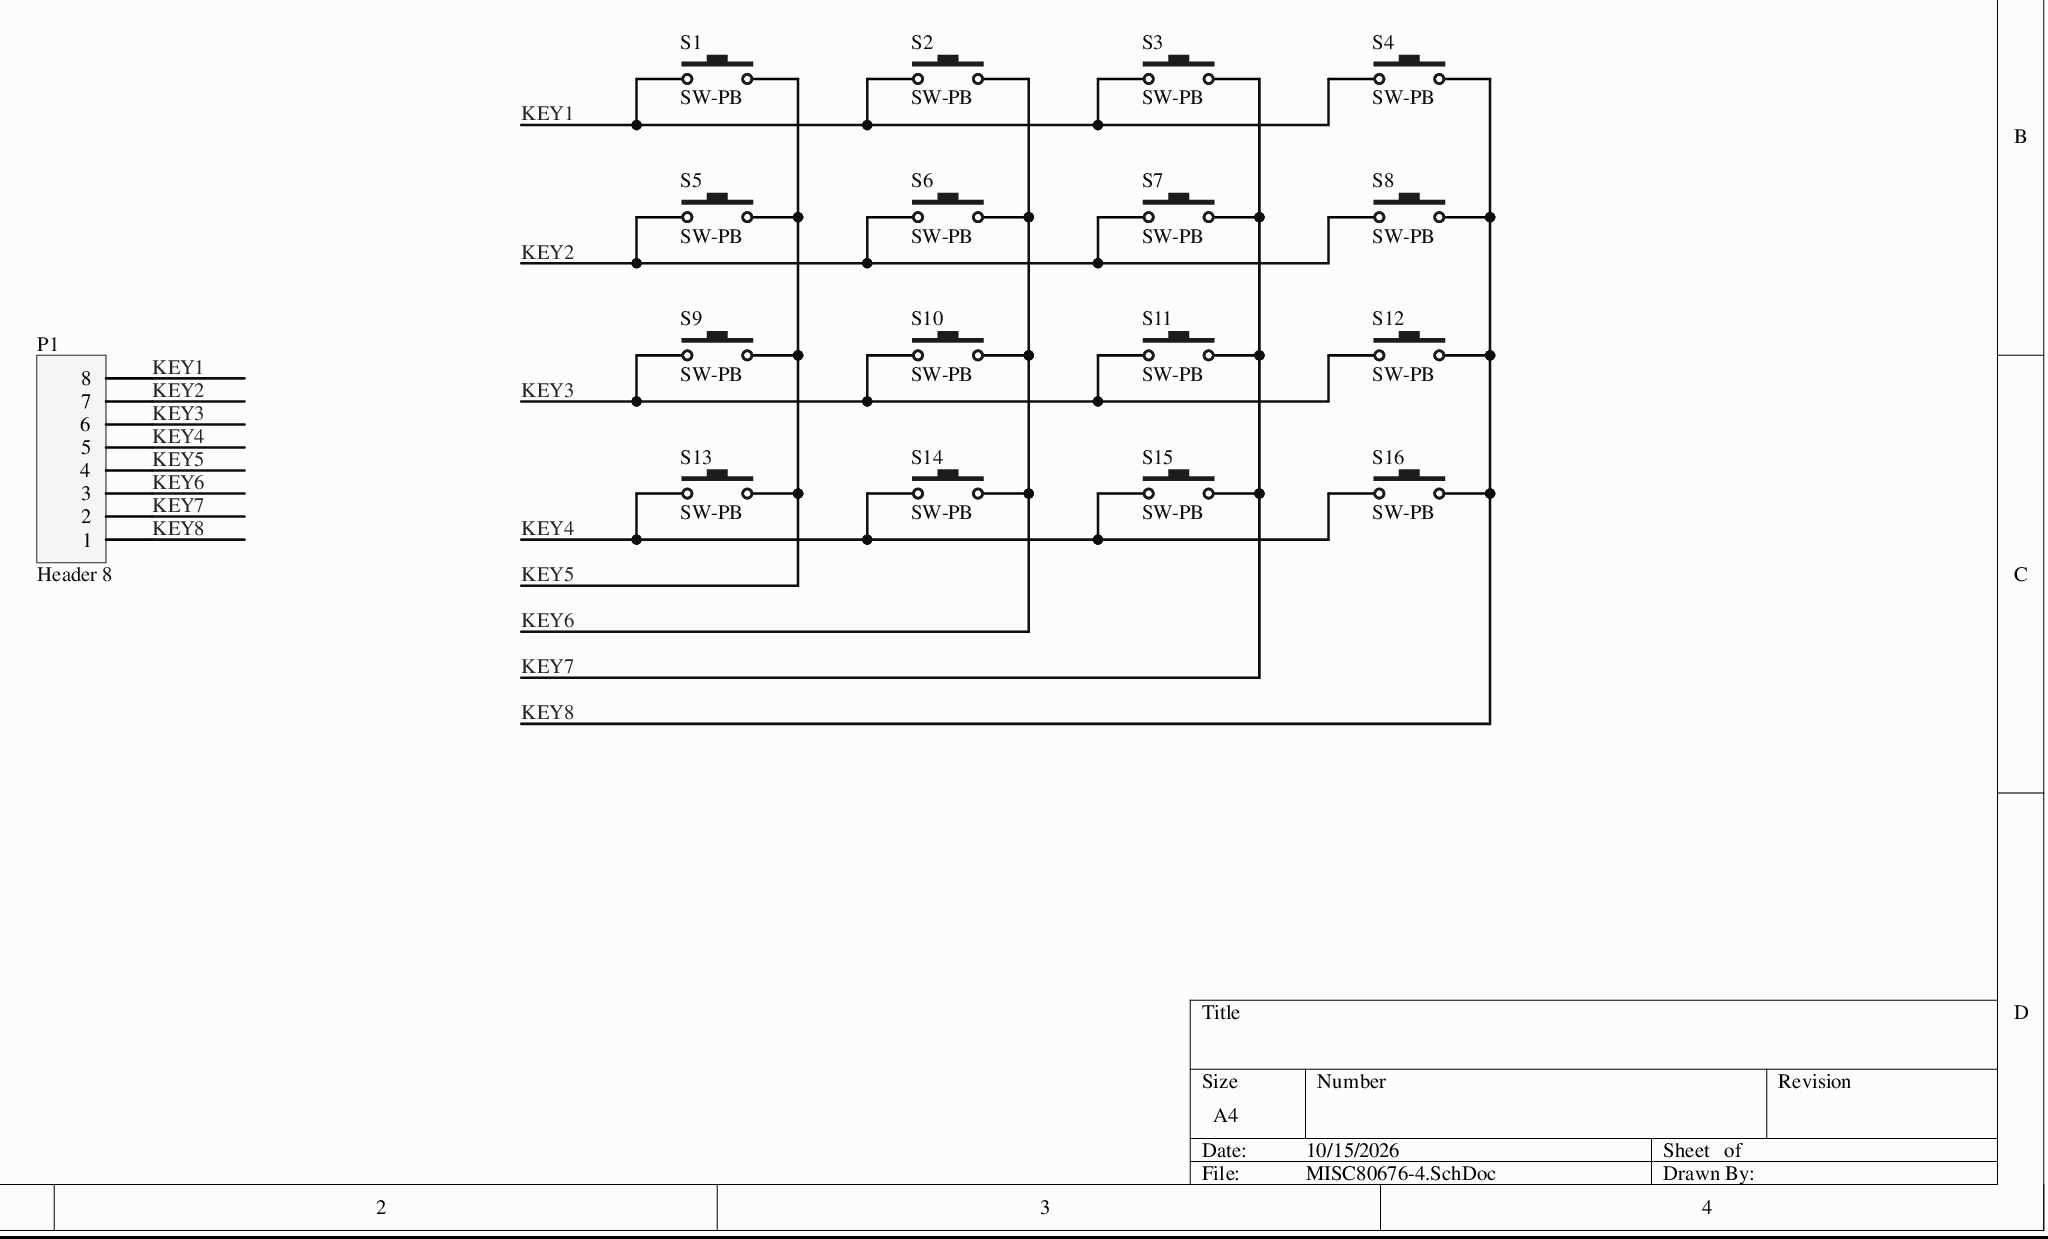
[diagram p0: MISC80676-4.SchDoc]
# Altium project MISC80676-7.PrjPcb
1 sheet, 17 parts. Net scope: global (net labels, ports and power ports of the same name join across sheets).
Board file: MISC80676.PcbDoc

## Sheet MISC80676-4.SchDoc
size A4

### Parts
P1  Header 8  [HDR1X8]
S1  SW-PB  [SPST-2]
S2  SW-PB  [SPST-2]
S3  SW-PB  [SPST-2]
S4  SW-PB  [SPST-2]
S5  SW-PB  [SPST-2]
S6  SW-PB  [SPST-2]
S7  SW-PB  [SPST-2]
S8  SW-PB  [SPST-2]
S9  SW-PB  [SPST-2]
S10  SW-PB  [SPST-2]
S11  SW-PB  [SPST-2]
S12  SW-PB  [SPST-2]
S13  SW-PB  [SPST-2]
S14  SW-PB  [SPST-2]
S15  SW-PB  [SPST-2]
S16  SW-PB  [SPST-2]

### Nets
KEY1: P1.8 S1.1 S2.1 S3.1 S4.1
KEY2: P1.7 S5.1 S6.1 S7.1 S8.1
KEY3: P1.6 S9.1 S10.1 S11.1 S12.1
KEY4: P1.5 S13.1 S14.1 S15.1 S16.1
KEY5: P1.4 S1.2 S5.2 S9.2 S13.2
KEY6: P1.3 S2.2 S6.2 S10.2 S14.2
KEY7: P1.2 S3.2 S7.2 S11.2 S15.2
KEY8: P1.1 S4.2 S8.2 S12.2 S16.2

### Library data of the parts
P1 = Header 8: Header, 8-Pin; LatestRevisionDate: 17-Jul-2002; LatestRevisionNote: Re-released for DXP Platform.; Publisher: COMPANY_A
S1-S16 = SW-PB: Switch; Published: 24-Mar-1999; LatestRevisionDate: 17-Jul-2002; LatestRevisionNote: Re-released for DXP Platform.; PackageReference: SPST-2; PackageDescription: Switch; 2 Leads; Publisher: COMPANY_A